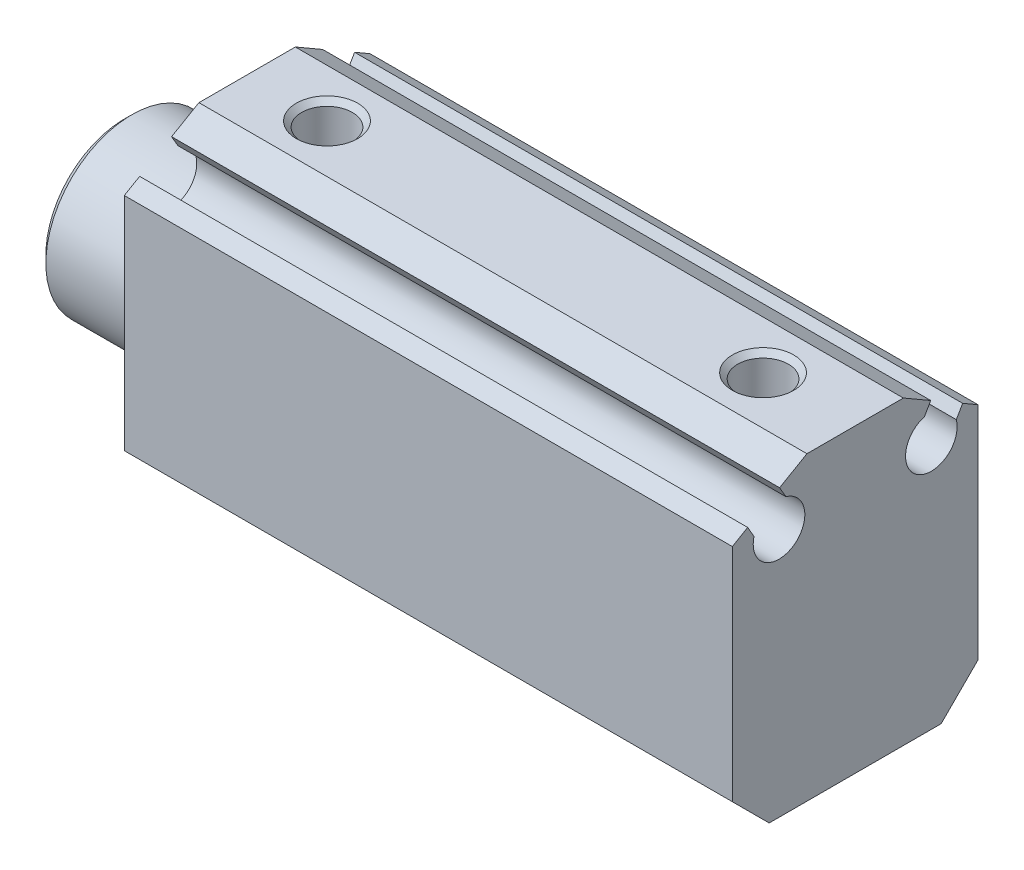
from build123d import *

# Parameters (mm, degrees)
BOSS_EXTRUDE1_DEPTH = 49.5


with BuildPart() as part:
    # Sketch1 → Boss-Extrude1 (new body)
    with BuildSketch(Plane(origin=(0, 0, 0), x_dir=(0, 0, -1), z_dir=(1, 0, 0))):
        with BuildLine():
            Line((-10, -7), (-7, -10))
            Line((-7, -10), (7, -10))
            Line((7, -10), (10, -7))
            Line((10, -7), (10, 10.992597115))
            Line((10, 10.992597115), (8.748941454, 11.714896103))
            Line((8.748941454, 11.714896103), (8.233885029, 10.822792206))
            ThreePointArc((8.233885029, 10.822792206), (5.15, 8.481346652), (5.635808817, 12.322792206))
            Line((5.635808817, 12.322792206), (6.150865242, 13.214896103))
            Line((6.150865242, 13.214896103), (3.925, 14.5))
            Line((3.925, 14.5), (-3.925, 14.5))
            Line((-3.925, 14.5), (-6.150865242, 13.214896103))
            Line((-6.150865242, 13.214896103), (-5.635808817, 12.322792206))
            ThreePointArc((-5.635808817, 12.322792206), (-5.15, 8.481346652), (-8.233885029, 10.822792206))
            Line((-8.233885029, 10.822792206), (-8.748941454, 11.714896103))
            Line((-8.748941454, 11.714896103), (-10, 10.992597115))
            Line((-10, 10.992597115), (-10, -7))
        make_face()
    extrude(amount=BOSS_EXTRUDE1_DEPTH)

    # Sketch2 → Revolve1 (revolve)
    with BuildSketch(Plane.XY, mode=Mode.PRIVATE) as revolve1_sk:
        Polygon((-10, 0), (-10, 6.3865), (-9.3865, 7), (0, 7), (0, 0), align=None)
    revolve(revolve1_sk.sketch.rotate(Axis((0, 0, 0), (-1, 0, 0)), 90), axis=Axis((0, 0, 0), (-1, 0, 0)))

    # Sketch3 → Cut-Revolve1 (revolve, cut)
    with BuildSketch(Plane.XY):
        Polygon((-10, 0), (-10, 3), (11, 3), (11, 8), (38.5, 8), (38.5, 0), align=None)
    revolve(axis=Axis((38.5, 0, 0), (-1, 0, 0)), mode=Mode.SUBTRACT)

    # Sketch4 → Cut-Revolve2 (revolve, cut)
    with BuildSketch(Plane.XY, mode=Mode.PRIVATE) as cut_revolve2_sk:
        Polygon((6.5, 14.5), (9, 14.5), (8.567, 14.067), (8.567, 8.5), (6.5, 7.2580211), align=None)
    revolve(cut_revolve2_sk.sketch.rotate(Axis((6.5, 7.2580211, 0), (0, 1, 0)), 90), axis=Axis((6.5, 7.2580211, 0), (0, 1, 0)), mode=Mode.SUBTRACT)

    # Sketch5 → Cut-Revolve3 (revolve, cut)
    with BuildSketch(Plane.XY, mode=Mode.PRIVATE) as cut_revolve3_sk:
        Polygon((42, 14.5), (44.5, 14.5), (44.067, 14.067), (44.067, 8.5), (42, 7.2580211), align=None)
    revolve(cut_revolve3_sk.sketch.rotate(Axis((42, 7.2580211, 0), (0, 1, 0)), 90), axis=Axis((42, 7.2580211, 0), (0, 1, 0)), mode=Mode.SUBTRACT)


solid = part.part
